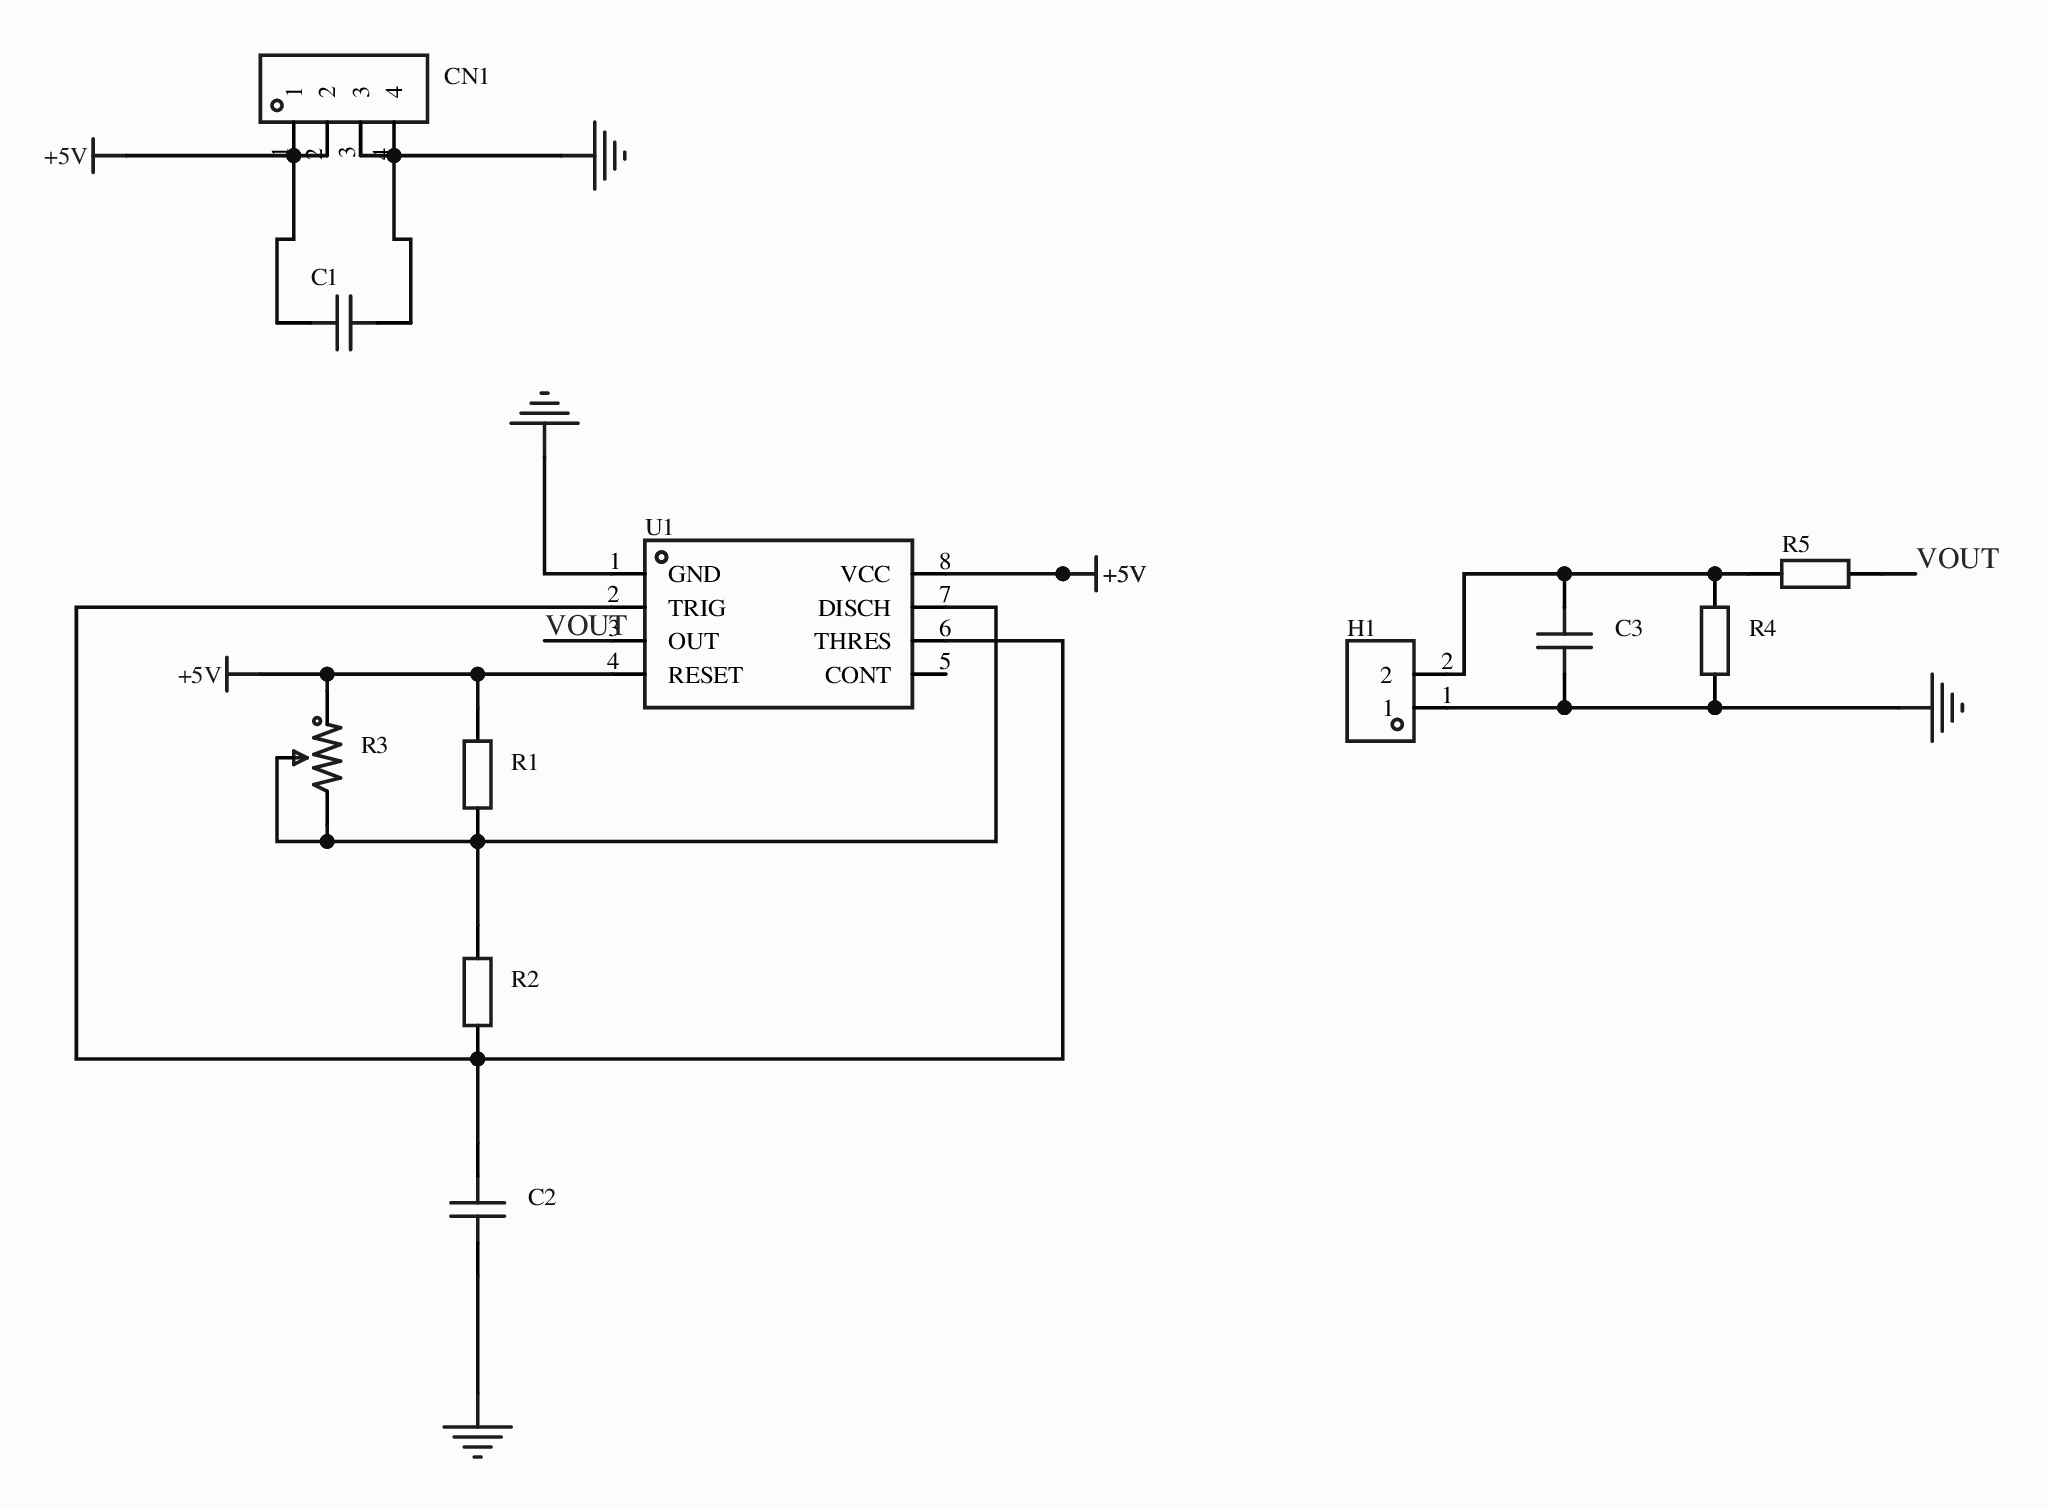
[diagram p0: MISC89121-3.schdoc]
# Altium project MISC89121-2.PrjPcb
1 sheet, 11 parts. Net scope: global (net labels, ports and power ports of the same name join across sheets).
Board file: MISC89121.pcbdoc

## Sheet MISC89121-3.schdoc
size 299 x 212 mm; Name: MISC89121

### Parts
C1  1uF  [C0805]  (value not drawn)
C2  10nF  [C0805]  (value not drawn)
C3  200pF  [C0805]  (value not drawn)
CN1  A2541WV-4P  [HDR-TH_4P-P2.54-V-M]  (value not drawn)
H1  A2541WV-2P  [HDR-TH_P2.54-H-M_A2541WV-2P]  (value not drawn)
R1  5kΩ  [R0805]  (value not drawn)
R2  3kΩ  [R0805]  (value not drawn)
R3  5kΩ  [RES-ADJ-TH_3P-L10.0-W10.0-P2.50-L]  (value not drawn)
R4  10kΩ  [R0805]  (value not drawn)
R5  10kΩ  [R0805]  (value not drawn)
U1  100kHz  [SOP-8_L5.0-W4.0-P1.27-LS6.0-BL]  (value not drawn)

### Nets
+5V: C1.2 CN1.1 CN1.2 R1.2 R3.1 U1.4(RESET) U1.8(VCC)
GND: C1.1 C2.1 C3.1 CN1.3 CN1.4 H1.1 R4.1 U1.1(GND)
VOUT: R5.2 U1.3(OUT)
NetC2_2: C2.2 R2.1 U1.2(TRIG) U1.6(THRES)
NetC3_2: C3.2 H1.2 R4.2 R5.1
NetR1_1: R1.1 R2.2 R3.2 R3.3 U1.7(DISCH)

Not connected (* = marked no-connect by the designer): U1 5(CONT)*

### Library data of the parts
C1 = 1uF: Capacitance: 22uF; Tolerance: ±20%; Rated voltage: 35V; Dielectric (temperature coefficient): X5R;; Manufacturer: HRE(芯声); Symbol: CGA0805X5R226M350MT; Add into BOM: yes; Origin Footprint: C0805; Device: 1uF; LCSC Part Name: 22uF ±20% 35V; Supplier Part: C6119901; Manufacturer Part: CGA0805X5R226M350MT; Supplier Footprint: 0805; JLCPCB Part Class: Extended library; Datasheet: https://atta.szlcsc.com/upload/public/pdf/source/20231129/D589D0CC4D260F7AC3A77E53B455CCB3.pdf; Supplier: LCSC; Convert to PCB: yes; Value: 1uF; Voltage Rated: 35V; Temperature Coefficient: X5R; FootprintName: C0805
C2 = 10nF: Capacitance: 22uF; Tolerance: ±20%; Rated voltage: 35V; Dielectric (temperature coefficient): X5R;; Manufacturer: HRE(芯声); Symbol: CGA0805X5R226M350MT; Add into BOM: yes; Origin Footprint: C0805; Device: 10nF; LCSC Part Name: 22uF ±20% 35V; Supplier Part: C6119901; Manufacturer Part: CGA0805X5R226M350MT; Supplier Footprint: 0805; JLCPCB Part Class: Extended library; Datasheet: https://atta.szlcsc.com/upload/public/pdf/source/20231129/D589D0CC4D260F7AC3A77E53B455CCB3.pdf; Supplier: LCSC; Convert to PCB: yes; Value: 10nF; Voltage Rated: 35V; Temperature Coefficient: X5R; FootprintName: C0805
C3 = 200pF: Capacitance: 200pF; Tolerance: ±5%; Rated voltage: 50V; Dielectric (temperature coefficient): NP0;; Manufacturer: YAGEO(国巨); Symbol: CC0805JRNPO9BN201; Add into BOM: yes; Origin Footprint: C0805; Device: 200pF; LCSC Part Name: 200pF ±5% 50V; Supplier Part: C520004; Manufacturer Part: CC0805JRNPO9BN201; Supplier Footprint: 0805; JLCPCB Part Class: Extended library; Datasheet: https://atta.szlcsc.com/upload/public/pdf/source/20200423/C520004_B99A110435D6B2A73BAACED9B50F0DDC.pdf; Supplier: LCSC; Convert to PCB: yes; Value: 200pF; Voltage Rated: 50V; Temperature Coefficient: NP0; FootprintName: C0805
CN1 = A2541WV-4P: Pin structure: 1x4P; Pitch: 2.54mm; Row spacing: -; Round/square pin: square pin; Mounting type: through-hole; Rows: single row; Total pins: 4P; Rated current: 3A; Rated voltage: 250V; Mating pin length: 6mm; Housing height: 2.54mm; Tail pin length: 3mm; Contact material: brass; Contact plating: gold; Operating temperature range: -40℃~+105℃; Color: black;; Manufacturer: CJT(长江连接器); Symbol: A2541WV-4P_C5346656; Add into BOM: yes; ModelId: 1d5b704bd9074887b1bc895e6ed65ccf; Origin Footprint: HDR-TH_4P-P2.54-V-M; Device: A2541WV-4P; LCSC Part Name: 1x4P 间距:2.54mm 方针 直插; Supplier Part: C5346656; Manufacturer Part: A2541WV-4P; Supplier Footprint: 插件,P=2.54mm; JLCPCB Part Class: Extended library; Datasheet: https://atta.szlcsc.com/upload/public/pdf/source/20210317/C225479_66BE1F584C1491F50F59A7D7B65E2652.pdf; Supplier: LCSC; Convert to PCB: yes; Pin Structure: 1x4P; Row Spacing: -; Circluar Pins/Square Pins: Square pin; Mounting Type: Through-hole; Number of Rows: Single row; Number of Pins: 4P; Current Rating (Max): 3A; Voltage Rating (Max): 250V; Length of Mating Pin: 6mm; Insulation Height: 2.54mm; Length of End Connection Pin: 3mm; Contact Material: Brass; Contact Plating: Gold; Operating Temperature Range: -40℃~+105℃; Color: Black; FootprintName: HDR-TH_4P-P2.54-V-M; ModelName: HDR-TH_4P-P2.54-V-M
H1 = A2541WV-2P: Pin structure: 1x2P; Pitch: 2.54mm; Row spacing: -; Round/square pin: square pin; Mounting type: through-hole; Rows: single row; Total pins: 2P; Rated current: 3A; Rated voltage: 250V; Mating pin length: 6mm; Housing height: 2.54mm; Tail pin length: 3mm; Contact material: brass; Contact plating: gold; Operating temperature range: -40℃~+105℃; Color: black;; Manufacturer: CJT(长江连接器); Symbol: A2541WV-2P_C225477; Add into BOM: yes; Origin Footprint: HDR-TH_P2.54-H-M_A2541WV-2P; Device: A2541WV-2P; LCSC Part Name: 1x2P 间距:2.54mm 方针 直插; Supplier Part: C225477; Manufacturer Part: A2541WV-2P; Supplier Footprint: 插件,P=2.54mm; JLCPCB Part Class: Extended library; Datasheet: https://atta.szlcsc.com/upload/public/pdf/source/20180724/C239359_48B1BC0CA1B4E4396A63955AAFD15564.pdf; Supplier: LCSC; Convert to PCB: yes; Pin Structure: 1x2P; Row Spacing: -; Circluar Pins/Square Pins: Square pin; Mounting Type: Through-hole; Number of Rows: Single row; Number of Pins: 2P; Current Rating (Max): 3A; Voltage Rating (Max): 250V; Length of Mating Pin: 6mm; Insulation Height: 2.54mm; Length of End Connection Pin: 3mm; Contact Material: Brass; Contact Plating: Gold; Operating Temperature Range: -40℃~+105℃; Color: Black; FootprintName: HDR-TH_P2.54-H-M_A2541WV-2P
R1 = 5kΩ: Resistor type: thick film resistor; Resistance: 10kΩ; Tolerance: ±5%; Power: 125mW; Max working voltage: 150V; Temperature coefficient: ±100ppm/℃;; Manufacturer: UNI-ROYAL(厚声); Symbol: 0805W8J0103T5E; Add into BOM: yes; ModelId: 1f8f9bfd8e2b427398b06535d781678a; Origin Footprint: R0805; Device: 5kΩ; LCSC Part Name: 10kΩ ±5% 125mW 厚膜电阻; Supplier Part: C25612; Manufacturer Part: 0805W8J0103T5E; Supplier Footprint: 0805; JLCPCB Part Class: Extended library; Datasheet: https://atta.szlcsc.com/upload/public/pdf/source/20200306/C422600_1E6D84923E4A46A82E41ADD87F860B5C.pdf; Supplier: LCSC; Convert to PCB: yes; Type: Thick film resistor; Value: 5kΩ; Power(Watts): 125mW; Overload Voltage (Max): 150V; Temperature Coefficient: ±100ppm/℃; Operating Temperature Range: -55℃~+155℃; FootprintName: R0805; ModelName: R0805
R2 = 3kΩ: Resistor type: thick film resistor; Resistance: 10kΩ; Tolerance: ±5%; Power: 125mW; Max working voltage: 150V; Temperature coefficient: ±100ppm/℃;; Manufacturer: UNI-ROYAL(厚声); Symbol: 0805W8J0103T5E; Add into BOM: yes; ModelId: 1f8f9bfd8e2b427398b06535d781678a; Origin Footprint: R0805; Device: 3kΩ; LCSC Part Name: 10kΩ ±5% 125mW 厚膜电阻; Supplier Part: C25612; Manufacturer Part: 0805W8J0103T5E; Supplier Footprint: 0805; JLCPCB Part Class: Extended library; Datasheet: https://atta.szlcsc.com/upload/public/pdf/source/20200306/C422600_1E6D84923E4A46A82E41ADD87F860B5C.pdf; Supplier: LCSC; Convert to PCB: yes; Type: Thick film resistor; Value: 3kΩ; Power(Watts): 125mW; Overload Voltage (Max): 150V; Temperature Coefficient: ±100ppm/℃; Operating Temperature Range: -55℃~+155℃; FootprintName: R0805; ModelName: R0805
R3 = 5kΩ: Resistance: 10kΩ; Tolerance: ±10%;; Manufacturer: BOCHEN(博晨); Symbol: 3296W-1-103; Add into BOM: yes; Origin Footprint: RES-ADJ-TH_3P-L10.0-W10.0-P2.50-L; Device: 5kΩ; LCSC Part Name: 10kΩ ±10%; Supplier Part: C118954; Manufacturer Part: 3296W-1-103; Supplier Footprint: 插件; JLCPCB Part Class: Extended library; Datasheet: https://atta.szlcsc.com/upload/public/pdf/source/20171114/C118954_15106326646611117443.pdf; Supplier: LCSC; Convert to PCB: yes; Value: 5kΩ; Tolerance: ±10%; FootprintName: RES-ADJ-TH_3P-L10.0-W10.0-P2.50-L
R4 R5 = 10kΩ: Resistor type: thick film resistor; Resistance: 10kΩ; Tolerance: ±1%; Power: 125mW; Max working voltage: 150V; Temperature coefficient: ±100ppm/℃;; Manufacturer: UNI-ROYAL(厚声); Manufacturer Part: 0805W8F1002T5E; Symbol: 0805W8F1002T5E_C17414; Add into BOM: yes; ModelId: 1f8f9bfd8e2b427398b06535d781678a; Origin Footprint: R0805; Device: 10kΩ; LCSC Part Name: 10kΩ ±1% 125mW 厚膜电阻; Supplier Part: C17414; Supplier Footprint: 0805; JLCPCB Part Class: Basic library; Datasheet: https://atta.szlcsc.com/upload/public/pdf/source/20200306/C422600_1E6D84923E4A46A82E41ADD87F860B5C.pdf; Supplier: LCSC; Convert to PCB: yes; Type: Thick film resistor; Value: 10kΩ; Power(Watts): 125mW; Overload Voltage (Max): 150V; Temperature Coefficient: ±100ppm/℃; Operating Temperature Range: -55℃~+155℃; FootprintName: R0805; ModelName: R0805
U1 = 100kHz: Frequency: 100kHz;; Manufacturer: UMW(友台半导体); Symbol: NE555DR; Add into BOM: yes; Supply Voltage: 4.5V~16V; Supply Current: 30nA; Origin Footprint: SOP-8_L5.0-W4.0-P1.27-LS6.0-BL; Device: 100kHz; LCSC Part Name: NE555DR; Supplier Part: C695838; Manufacturer Part: NE555DR; Supplier Footprint: SOP-8; JLCPCB Part Class: Extended library; Datasheet: https://atta.szlcsc.com/upload/public/pdf/source/20231109/10F1BB7F0C3DC760A85BC3699079301C.pdf; Supplier: LCSC; Convert to PCB: yes; Value: 100kHz; Operating Temperature: 0℃~+70℃; FootprintName: SOP-8_L5.0-W4.0-P1.27-LS6.0-BL